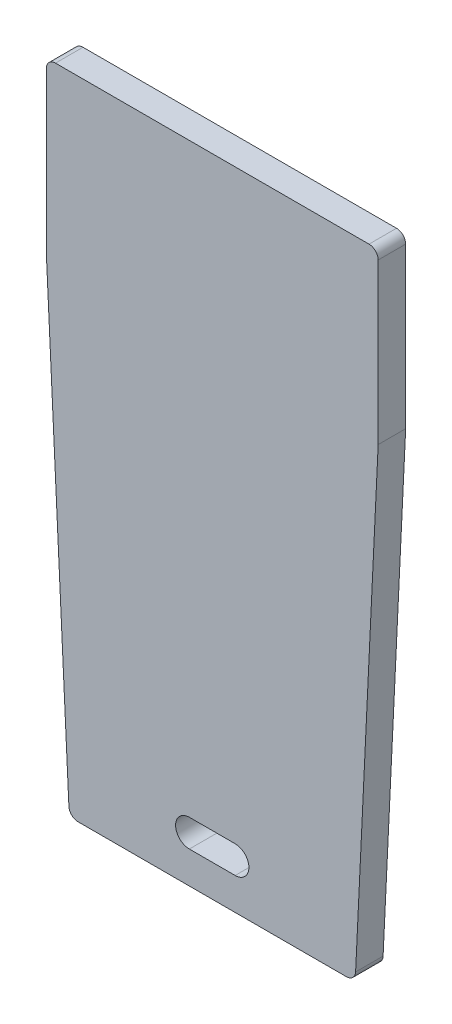
SolidWorks part; units mm, degrees
material "普通碳钢"
ref_plane "Front Plane" through (0, 0, 0) normal (0, 0, 1) x (1, 0, 0)
ref_plane "Top Plane" through (0, 0, 0) normal (0, 1, 0) x (1, 0, 0)
ref_plane "Right Plane" through (0, 0, 0) normal (1, 0, 0) x (0, 0, -1)
sketch "Sketch1" plane through (0, 0, 0) normal (0, 0, 1) x (1, 0, 0)
  line L0 (0, 579.2516) -> (0, -304.1584) construction
  line L1 (108.65, 415.8) -> (-108.65, 415.8)
  line L2 (-115, 409.45) -> (-115, 298.68)
  line L3 (-115, 298.68) -> (-99.3516, -25.706)
  line L4 (-93.0089, -31.75) -> (93.0089, -31.75)
  line L5 (-15.875, 0) -> (15.875, 0) construction
  line L6 (-15.875, 9.525) -> (15.875, 9.525)
  line L7 (-15.875, -9.525) -> (15.875, -9.525)
  line L8 (115, 298.68) -> (99.3516, -25.706)
  line L9 (115, 409.45) -> (115, 298.68)
  arc A0 (-15.875, 9.525) -> (-15.875, -9.525) centre (-15.875, 0) ccw
  arc A1 (15.875, -9.525) -> (15.875, 9.525) centre (15.875, 0) ccw
  arc A2 (-99.3516, -25.706) -> (-93.0089, -31.75) centre (-93.0089, -25.4) ccw
  arc A3 (-108.65, 415.8) -> (-115, 409.45) centre (-108.65, 409.45) ccw
  arc A4 (108.65, 415.8) -> (115, 409.45) centre (108.65, 409.45) cw
  arc A5 (99.3516, -25.706) -> (93.0089, -31.75) centre (93.0089, -25.4) cw
  point P10 (0, 0)
  point P17 (-99.06, -31.75)
  point P20 (-115, 415.8)
  point P22 (0, -31.75)
  point P23 (0, 415.8)
  point P28 (115, 415.8)
  point P29 (99.06, -31.75)
  dimension "D7" = 9.525
  dimension "D8" = 6.35
  dimension "D1" = 31.75
  dimension "D2" = 447.55
  dimension "D3" = 117.12
  dimension "D4" = 115
  dimension "D5" = 99.06
  dimension "D6" = 31.75
extrude "Boss-Extrude1" add sketch "Sketch1" along normal mid plane 19.05
